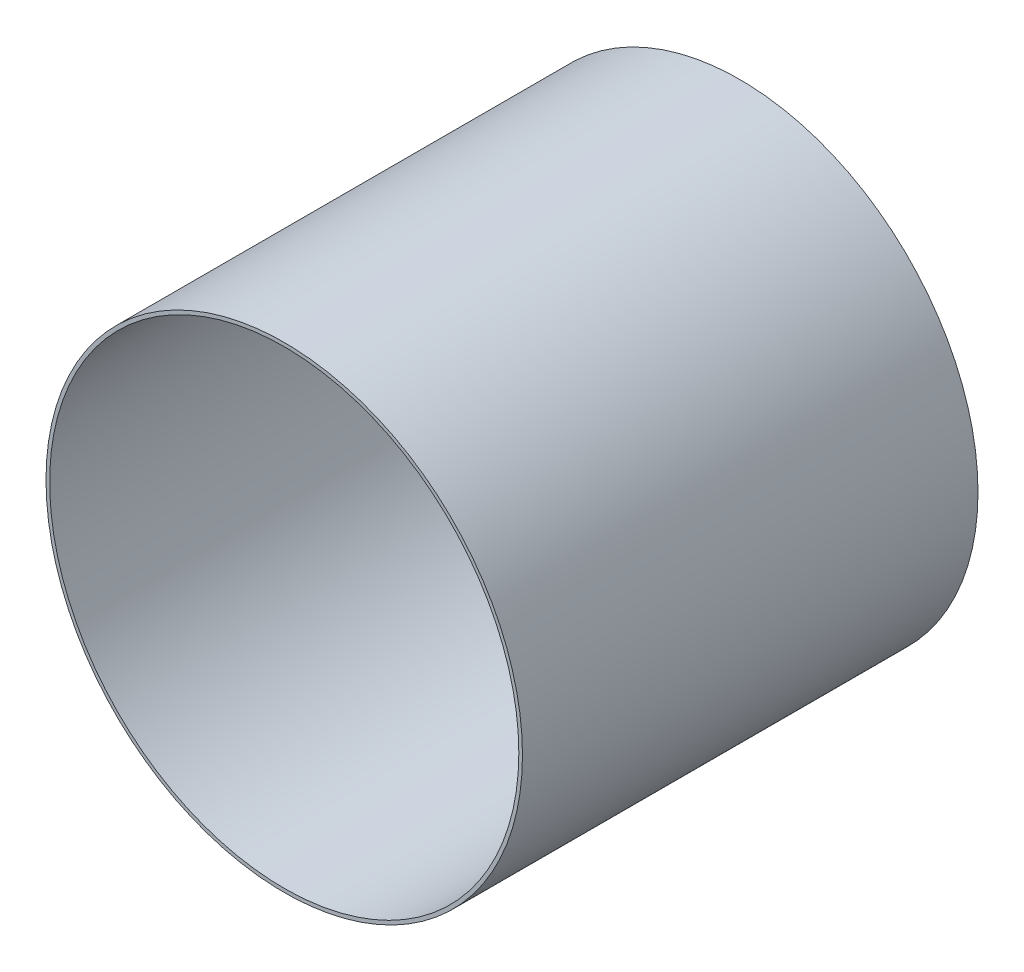
from build123d import *

# Parameters (mm, degrees)
SKETCH1_R           = 523
SKETCH1_R_2         = 515
EXTRUDE_THIN1_DEPTH = 500


with BuildPart() as part:
    # Sketch1 → Extrude-Thin1 (new, symmetric)
    with BuildSketch(Plane.XY):
        Circle(SKETCH1_R)
        Circle(SKETCH1_R_2, mode=Mode.SUBTRACT)
    extrude(amount=EXTRUDE_THIN1_DEPTH, both=True)


solid = part.part
